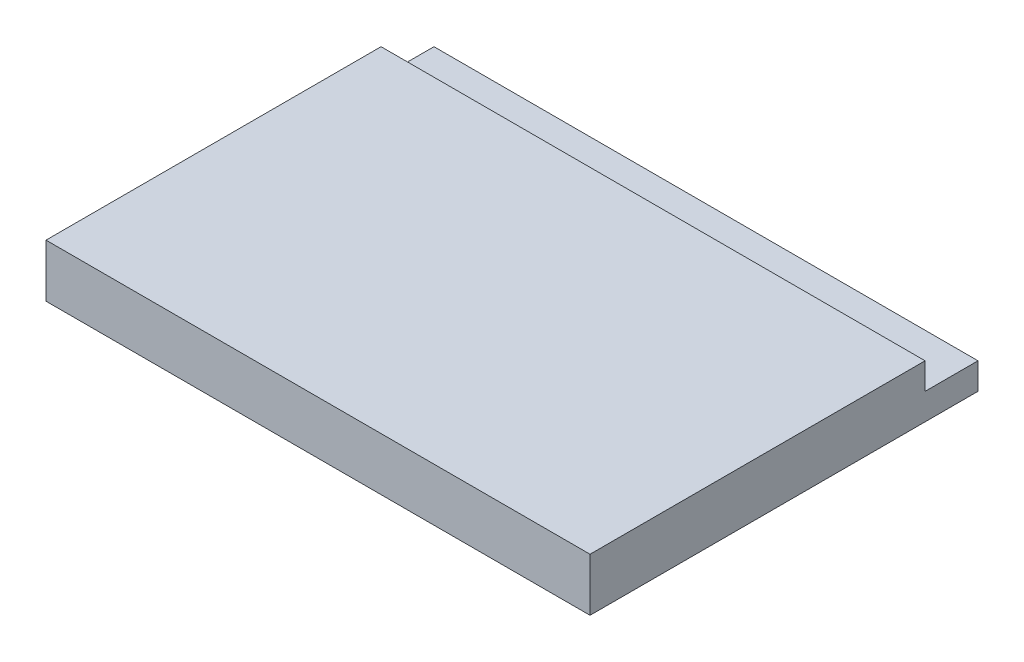
SolidWorks part; units mm, degrees
ref_plane "前视基准面" through (0, 0, 0) normal (0, 0, 1) x (1, 0, 0)
ref_plane "上视基准面" through (0, 0, 0) normal (0, 1, 0) x (1, 0, 0)
ref_plane "右视基准面" through (0, 0, 0) normal (1, 0, 0) x (0, 0, -1)
sketch "草图1" plane through (0, 0, 0) normal (0, 1, 0) x (1, 0, 0)
  line L1 (-154.25, -110) -> (154.25, -110)
  line L2 (-154.25, -110) -> (-154.25, 110)
  line L3 (-154.25, 110) -> (154.25, 110)
  line L4 (154.25, -110) -> (154.25, 110)
  line L5 (-154.25, -110) -> (154.25, 110) construction
  line L6 (-154.25, 110) -> (154.25, -110) construction
  point P0 (0, 0)
  dimension "D1" = 308.5
  dimension "D2" = 220
extrude "凸台-拉伸1" add sketch "草图1" along normal blind 30
sketch "草图2" plane through (0, 30, 0) normal (0, 1, 0) x (1, 0, 0)
  line L0 (154.25, 110) -> (-154.25, 110) construction
  line L1 (-167.4542, 80) -> (199.0088, 80)
  line L2 (-167.4542, 80) -> (-167.4542, 148.1692)
  line L3 (-167.4542, 148.1692) -> (199.0088, 148.1692)
  line L4 (199.0088, 80) -> (199.0088, 148.1692)
  dimension "D1" = 30
extrude "切除-拉伸1" cut sketch "草图2" against normal blind 15
